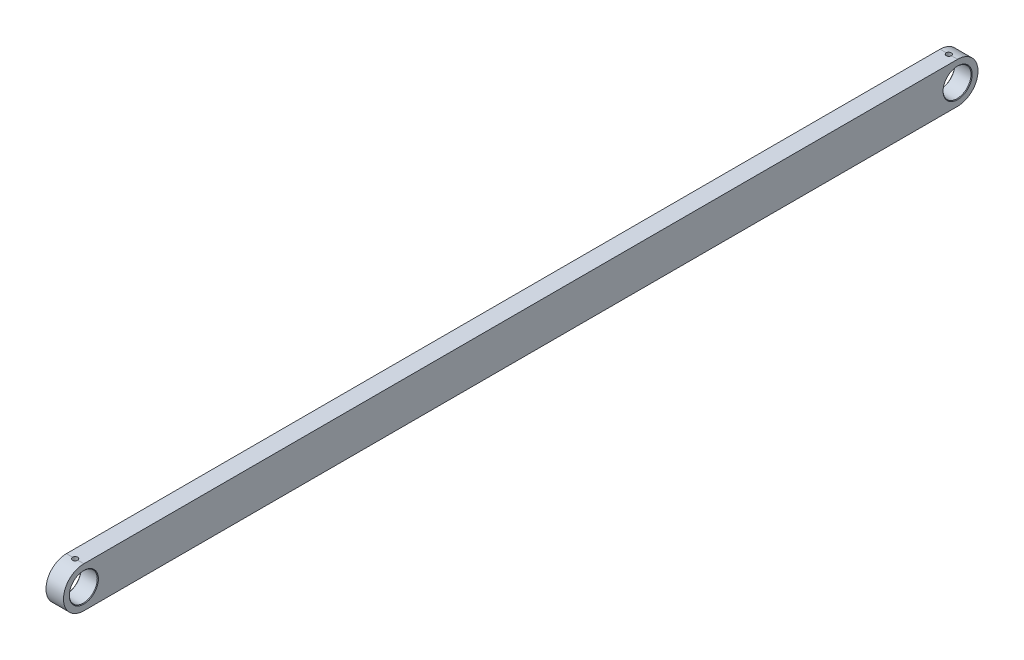
SolidWorks part; units mm, degrees
material "1.7131 (16MnCr5)"
ref_plane "前视基准面" through (0, 0, 0) normal (0, 0, 1) x (1, 0, 0)
ref_plane "上视基准面" through (0, 0, 0) normal (0, 1, 0) x (1, 0, 0)
ref_plane "右视基准面" through (0, 0, 0) normal (1, 0, 0) x (0, 0, -1)
sketch "草图1" plane through (0, 0, 0) normal (1, 0, 0) x (0, 0, -1)
  line L0 (-214.4997, 0) -> (182.531, 0) construction
  line L1 (0, 429.6355) -> (0, -56.0826) construction
  line L2 (-750, -35) -> (750, -35)
  line L4 (-750, 35) -> (750, 35)
  circle A0 centre (-750, 0) radius 24
  circle A1 centre (750, 0) radius 24
  arc A2 (-750, 35) -> (-750, -35) centre (-750, 0) ccw
  arc A3 (750, 35) -> (750, -35) centre (750, 0) cw
  dimension "D2" = 48
  dimension "D5" = 35
  dimension "D1" = 1500
extrude "凸台-拉伸1" add sketch "草图1" along normal mid plane 30
hole_wizard "M10x1.0 螺纹孔1" positions "草图3" profile "草图2" tap size "M10x1.0" standard "GB"
sketch "草图3" plane through (0, 35, 0) normal (0, 1, 0) x (1, 0, 0)
  line L0 (-157.5397, 0) -> (149.4319, 0) construction
  line L2 (0, 141.4603) -> (0, -127.4098) construction
  point P0 (0, -750)
  point P2 (0, 750)
  dimension "D1" = 1500
sketch "草图2" plane through (0, 35, 750) normal (1, 0, 0) x (0, 0, 1)
  line L0 (0, 0) -> (0, 22.7039)
  line L1 (0, 22.7039) -> (4.5, 20)
  line L2 (4.5, 20) -> (4.5, 0)
  line L5 (4.5, 0) -> (0, 0)
  line L10 (0, 22.7039) -> (-4.5, 20) construction
  line L11 (0, -6.35) -> (0, 107.95) construction
  dimension "螺纹孔钻头直径" = 9
  dimension "螺纹孔钻头深度" = 20
  dimension "导头角度" = 118
cosmetic thread "孔螺蚊线3" parameters "D1"=10, "D2"=10
cosmetic thread "孔螺蚊线4" parameters "D1"=10, "D2"=10
chamfer "倒角1" distance 1 angle 45 4 edges at (15, 0, -774) (-15, 0, -774) (-15, 0, 726) (15, 0, 726)
